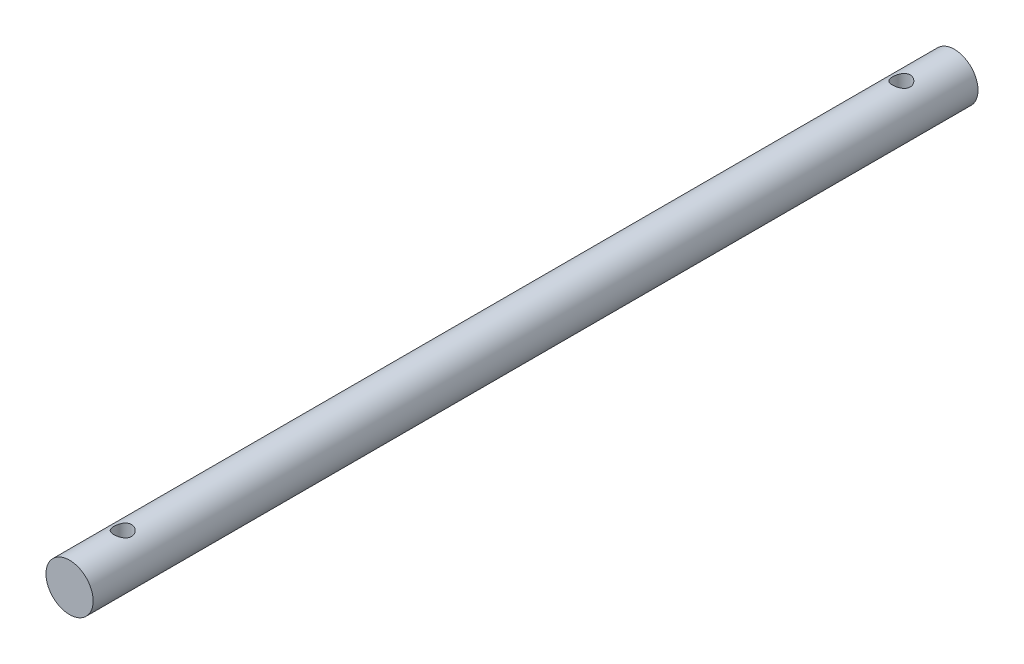
from build123d import *

# Parameters (mm, degrees)
SKETCH1_R           = 4
BOSS_EXTRUDE1_DEPTH = 75
SKETCH3_R           = 1.5
CUT_EXTRUDE1_DEPTH  = 5


with BuildPart() as part:
    # Sketch1 → Boss-Extrude1 (new, symmetric)
    with BuildSketch(Plane.XY):
        Circle(SKETCH1_R)
    extrude(amount=BOSS_EXTRUDE1_DEPTH, both=True)

    # Sketch3 → Cut-Extrude1 (cut, symmetric)
    with BuildSketch(Plane(origin=(0, 0, 0), x_dir=(1, 0, 0), z_dir=(0, 1, 0))):
        with Locations(Location((0, 66, 0), (0, 0, 270))):
            Circle(SKETCH3_R)
        with Locations(Location((0, -66, 0), (0, 0, 270))):
            Circle(SKETCH3_R)
    extrude(amount=CUT_EXTRUDE1_DEPTH, both=True, mode=Mode.SUBTRACT)


solid = part.part
